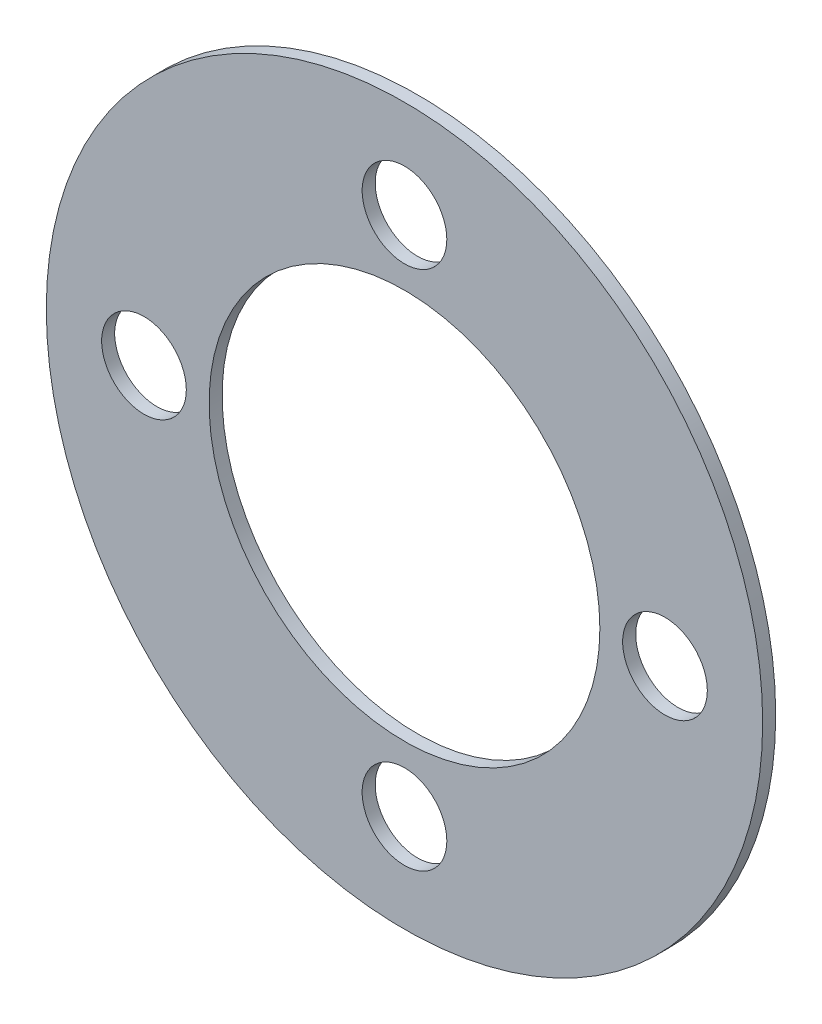
from build123d import *

# Parameters (mm, degrees)
SKETCH1_R           = 27.5
SKETCH1_R_2         = 15
SKETCH1_R_3         = 3.25
BOSS_EXTRUDE1_DEPTH = 1


with BuildPart() as part:
    # Sketch1 → Boss-Extrude1 (new body)
    with BuildSketch(Plane.XY):
        Circle(SKETCH1_R)
        Circle(SKETCH1_R_2, mode=Mode.SUBTRACT)
        with Locations((0, 20)):
            Circle(SKETCH1_R_3, mode=Mode.SUBTRACT)
        with Locations((20, 0)):
            Circle(SKETCH1_R_3, mode=Mode.SUBTRACT)
        with Locations((0, -20)):
            Circle(SKETCH1_R_3, mode=Mode.SUBTRACT)
        with Locations((-20, 0)):
            Circle(SKETCH1_R_3, mode=Mode.SUBTRACT)
    extrude(amount=BOSS_EXTRUDE1_DEPTH)


solid = part.part
